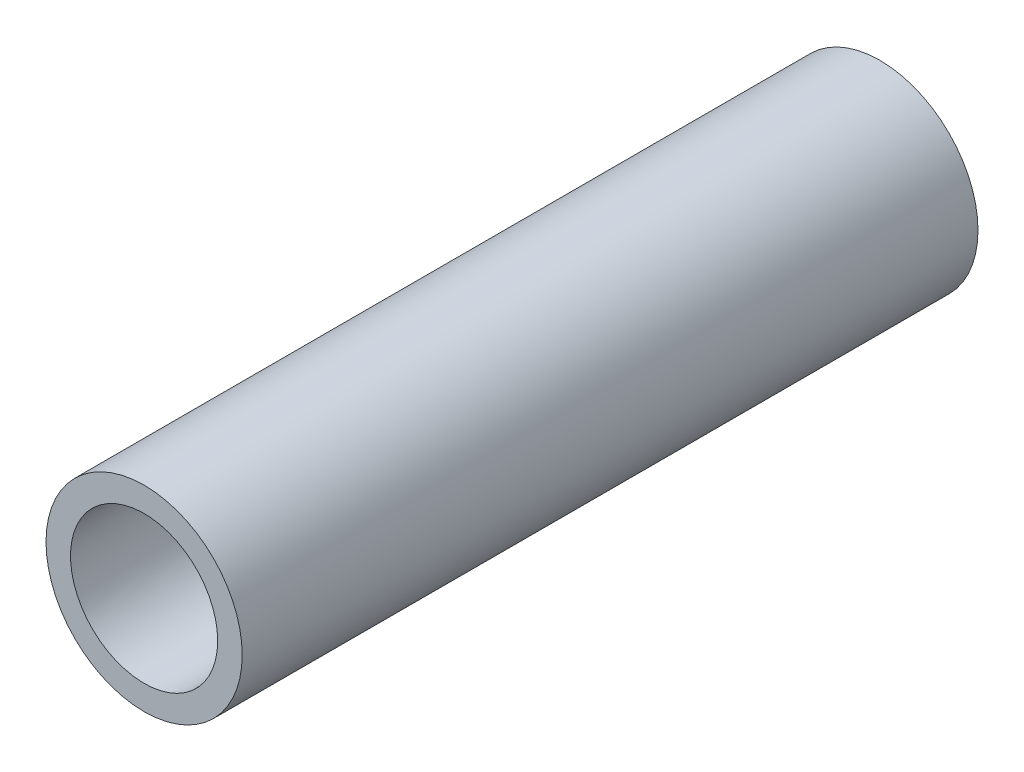
SolidWorks part; units mm, degrees
ref_plane "前视基准面" through (0, 0, 0) normal (0, 0, 1) x (1, 0, 0)
ref_plane "上视基准面" through (0, 0, 0) normal (0, 1, 0) x (1, 0, 0)
ref_plane "右视基准面" through (0, 0, 0) normal (1, 0, 0) x (0, 0, -1)
sketch "草图1" plane through (0, 0, 0) normal (0, 0, 1) x (1, 0, 0)
  circle A0 centre (0, 0) radius 8
  circle A1 centre (0, 0) radius 6
  dimension "D1" = 16
  dimension "D2" = 2
extrude "凸台-拉伸1" add sketch "草图1" along normal blind 60
